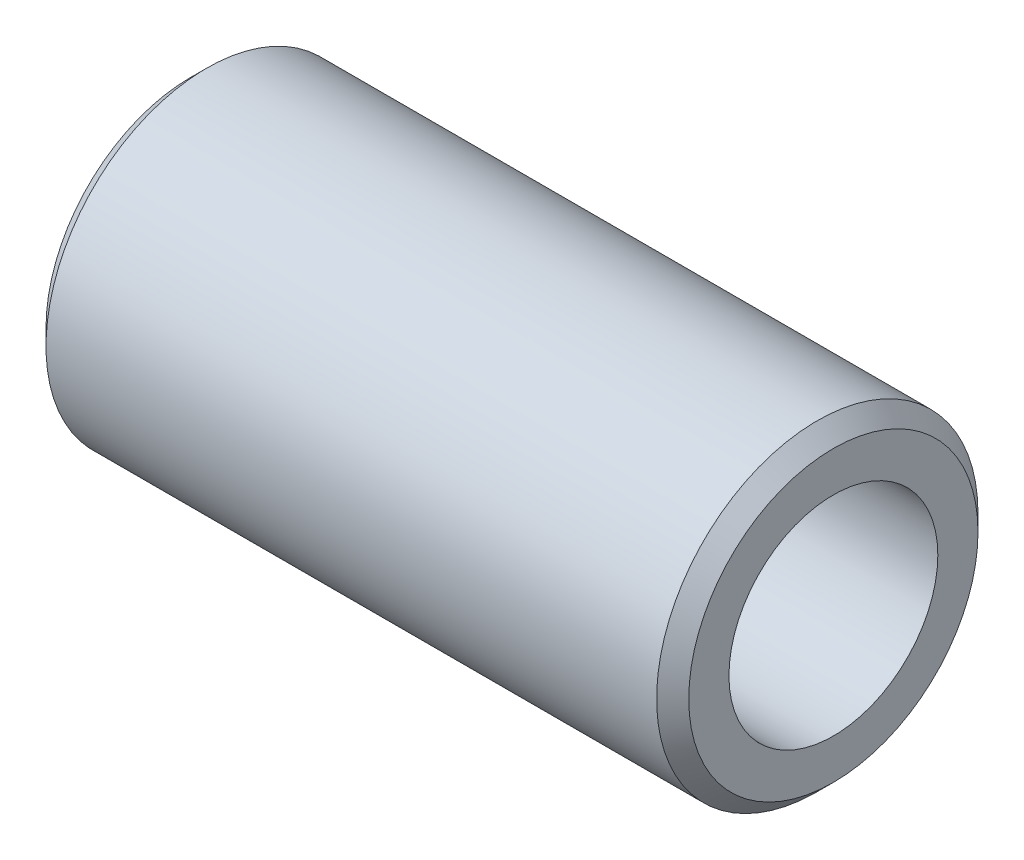
SolidWorks part; units mm, degrees
material "45#"
ref_plane "Front" through (0, 0, 0) normal (0, 0, 1) x (1, 0, 0)
ref_plane "Top" through (0, 0, 0) normal (0, 1, 0) x (1, 0, 0)
ref_plane "Right" through (0, 0, 0) normal (1, 0, 0) x (0, 0, -1)
sketch "草图1" plane through (0, 0, 0) normal (1, 0, 0) x (0, 0, -1)
  circle A0 centre (0, 0) radius 5
  dimension "D1" = 10
extrude "凸台-拉伸1" add sketch "草图1" along normal blind 20
chamfer "倒角1" distance 0.5 angle 45 2 edges at (0, 0, -5) (20, 0, -5)
sketch "草图2" plane through (0, 0, 0) normal (-1, 0, 0) x (0, 0, 1)
  circle A0 centre (0, 0) radius 3.25
  dimension "D1" = 6.5
extrude "切除-拉伸1" cut sketch "草图2" against normal through all
